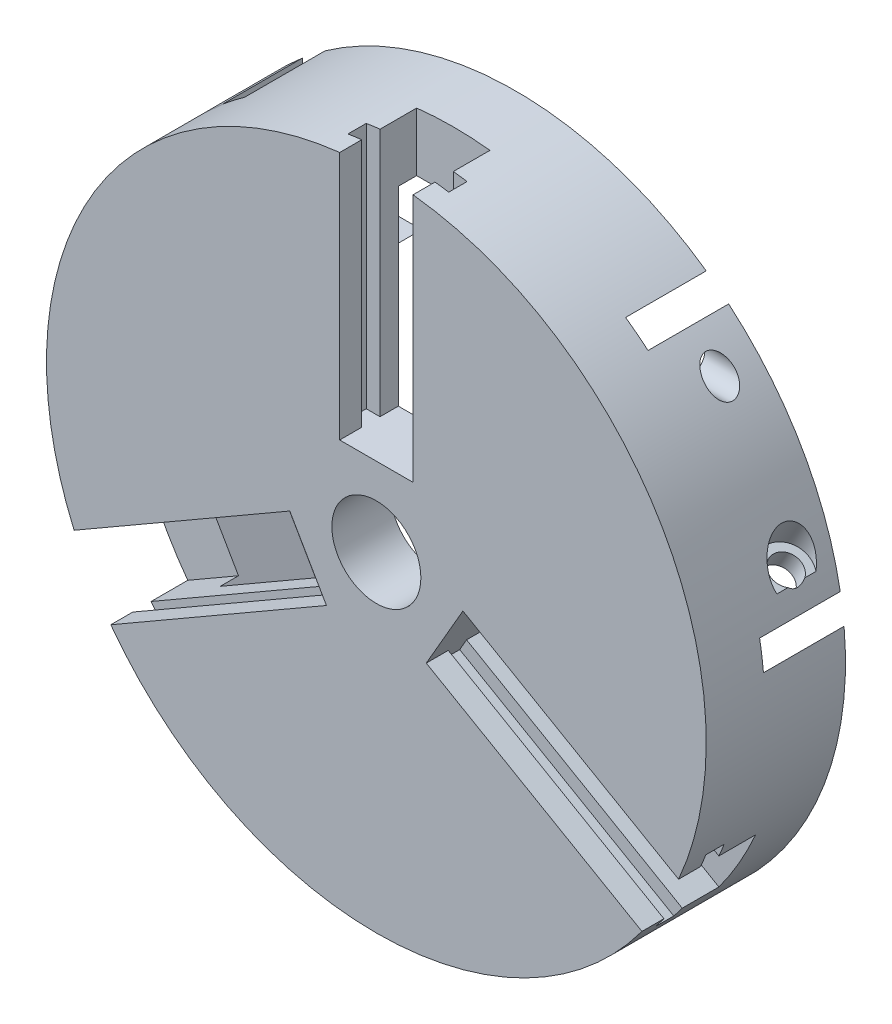
SolidWorks part; units mm, degrees
ref_plane "Front Plane" through (0, 0, 0) normal (0, 0, 1) x (1, 0, 0)
ref_plane "Top Plane" through (0, 0, 0) normal (0, 1, 0) x (1, 0, 0)
ref_plane "Right Plane" through (0, 0, 0) normal (1, 0, 0) x (0, 0, -1)
sketch "Sketch1" plane through (0, 0, 0) normal (0, 0, 1) x (1, 0, 0)
  circle A0 centre (0, 0) radius 180
  dimension "D1" = 360
extrude "Boss-Extrude1" add sketch "Sketch1" along normal blind 32
sketch "Sketch2" plane through (0, 0, 32) normal (0, 0, 1) x (1, 0, 0)
  line L0 (0, 188.4796) -> (0, 43) construction
  line L1 (20, 187.4154) -> (20, 43)
  line L2 (-20, 187.4154) -> (-20, 43)
  line L3 (-20, 43) -> (20, 43)
  arc A2 (20, 187.4154) -> (-20, 187.4154) centre (0, 0) ccw
  point P1 (0, 43)
  point P7 (0, 92.5)
  dimension "D1" = 43
  dimension "D3" = 40
extrude "Cut-Extrude1" cut sketch "Sketch2" against normal blind 40
pattern_circular "CirPattern1" count 3 over 360 about axis through (0, 0, 0) along (0, 0, 1) of "Cut-Extrude1"
sketch "Sketch3" plane through (37.2391, -21.5, 0) normal (0.866, -0.5, 0) x (0, 0, -1)
  line L0 (0, 0) -> (-32, 0) construction
  line L1 (-32, 20) -> (-32, -20) construction
  line L3 (-20, 27.5) -> (-10, 27.5)
  line L4 (-20, 27.5) -> (-20, -27.5)
  line L5 (-20, -27.5) -> (-10, -27.5)
  line L6 (-10, 27.5) -> (-10, -27.5)
  line L7 (-20, 27.5) -> (-10, -27.5) construction
  line L8 (-20, -27.5) -> (-10, 27.5) construction
  line L9 (0, 20) -> (0, 180) construction
  point P5 (-15, 0)
  dimension "D1" = 55
  dimension "D2" = 10
  dimension "D3" = 10
extrude "Cut-Extrude2" cut sketch "Sketch3" along normal blind 160
pattern_circular "CirPattern2" count 3 over 360 about axis through (0, 0, 0) along (0, 0, 1) of "Cut-Extrude2"
extrude "Cut-Extrude3" cut sketch "Sketch4" against normal blind 1
sketch "Sketch4" plane through (1185.0544, -482.7132, 0) normal (0, 0, -1) x (1, 0, 0)
  line L0 (-1236.3044, -571.4808) -> (-1301.3044, -571.4808)
  line L1 (-1301.3044, -571.4808) -> (-1301.3044, -620.1393)
  line L4 (-1133.8044, -571.4808) -> (-1068.8044, -571.4808)
  line L5 (-1068.8044, -571.4808) -> (-1068.8044, -620.1393)
  line L6 (-1301.3044, -620.1393) -> (-1068.8044, -620.1393) construction
  line L7 (-1236.3044, -393.9456) -> (-1203.8044, -337.6539)
  line L8 (-1203.8044, -337.6539) -> (-1245.9439, -313.3247)
  line L9 (-1287.5544, -482.7132) -> (-1320.0544, -539.0048)
  line L10 (-1320.0544, -539.0048) -> (-1362.1939, -514.6756)
  line L11 (-1082.5544, -482.7132) -> (-1050.0544, -539.0048)
  line L12 (-1050.0544, -539.0048) -> (-1007.9149, -514.6756)
  line L13 (-1133.8044, -393.9456) -> (-1166.3044, -337.6539)
  line L14 (-1166.3044, -337.6539) -> (-1124.1649, -313.3247)
  line L15 (-1236.3044, -571.4808) -> (-1185.0544, -482.7132) construction
  line L16 (-1185.0544, -482.7132) -> (-1133.8044, -571.4808) construction
  arc A0 (-1133.8044, -571.4808) -> (-1082.5544, -482.7132) centre (-1185.0544, -482.7132) ccw
  arc A1 (-1362.1939, -514.6756) -> (-1301.3044, -620.1393) centre (-1185.0544, -482.7132) ccw
  arc A4 (-1124.1649, -313.3247) -> (-1245.9439, -313.3247) centre (-1185.0544, -482.7132) ccw
  arc A5 (-1068.8044, -620.1393) -> (-1007.9149, -514.6756) centre (-1185.0544, -482.7132) ccw
  arc A6 (-1287.5544, -482.7132) -> (-1236.3044, -571.4808) centre (-1185.0544, -482.7132) ccw
  arc A7 (-1133.8044, -393.9456) -> (-1236.3044, -393.9456) centre (-1185.0544, -482.7132) ccw
sketch "Sketch5" plane through (0, 0, 0) normal (0, 0, -1) x (-1, 0, 0)
  line L0 (-116.25, 137.4261) -> (-116.25, 88.7676)
  line L1 (-102.5, 0) -> (-135, 56.2917)
  line L2 (-135, 56.2917) -> (-177.1395, 31.9624)
  line L3 (-116.25, 88.7676) -> (-51.25, 88.7676)
  arc A1 (-116.25, 137.4261) -> (-177.1395, 31.9624) centre (0, 0) ccw
  arc A2 (-51.25, 88.7676) -> (-102.5, 0) centre (0, 0) ccw
  arc A3 (-20, 178.8854) -> (-116.25, 137.4261) centre (0, 0) ccw construction
extrude "Boss-Extrude2" add sketch "Sketch5" along normal blind 44 and the other way blind 1 separate body
pattern_circular "CirPattern5" count 3 over 360 about axis through (0, 0, 0) along (0, 0, 1) of bodies 107
sketch "Sketch6" plane through (58.125, 100.6755, 0) normal (-0.5, -0.866, 0) x (0.866, -0.5, 0)
  line L0 (0, -23) -> (121.75, -23) construction
  line L1 (31.9624, -44) -> (137.4261, -44) construction
  circle A0 centre (121.75, -23) radius 8
  dimension "D3" = 16
  dimension "D1" = 121.75
  dimension "D2" = 21
extrude "Cut-Extrude4" cut sketch "Sketch6" against normal blind 51 and the other way blind 281
pattern_circular "CirPattern6" count 3 over 360 about axis through (0, 0, 32) along (0, 0, -1) of "Cut-Extrude4"
ref_plane "Plane1" through (63.125, -109.3357, 0) normal (-0.5, 0.866, 0) x (0.866, 0.5, 0)
sketch "Sketch7" plane through (63.125, -109.3357, 0) normal (-0.5, 0.866, 0) x (0.866, 0.5, 0)
  circle A0 centre (-121.75, 23) radius 12.5
  dimension "D1" = 25
extrude "Cut-Extrude5" cut sketch "Sketch7" against normal blind 30
pattern_circular "CirPattern7" count 3 over 360 about axis through (0, 0, 0) along (0, 0, 1) of "Cut-Extrude5"
sketch "Sketch10" plane through (0, 0, 0) normal (0, 0, -1) x (-1, 0, 0)
  line L0 (-179.2321, 16.6092) -> (-75.2321, -163.5241)
  line L1 (-47.2391, -4.1795) -> (-27.2391, -38.8205) construction
  line L2 (104, 146.9149) -> (-104, 146.9149)
  line L3 (75.2321, -163.5241) -> (179.2321, 16.6092)
  arc A0 (-177.1395, 31.9624) -> (-164.9193, -72.1222) centre (0, 0) ccw construction
  arc A1 (-144.9193, -106.7632) -> (-60.8895, -169.3885) centre (0, 0) ccw construction
  arc A2 (-179.2321, 16.6092) -> (-75.2321, -163.5241) centre (0, 0) ccw
  arc A3 (104, 146.9149) -> (-104, 146.9149) centre (0, 0) ccw
  arc A4 (75.2321, -163.5241) -> (179.2321, 16.6092) centre (0, 0) ccw
  point P17 (0, 0)
  dimension "D1" = 208
  dimension "D2" = 3
extrude "Boss-Extrude3" add sketch "Sketch10" along normal up to surface (44 mm away) up to face at (119.912, 69.2312, -44)
sketch "Sketch11" plane through (-37.2391, -21.5, 0) normal (-0.866, -0.5, 0) x (0, 0, 1)
  line L0 (0, -20) -> (10, -20) construction
  line L1 (0, 20) -> (-10, 20)
  line L2 (0, 20) -> (0, -20)
  line L3 (0, -20) -> (-10, -20)
  line L4 (-10, 20) -> (-10, -20)
  dimension "D1" = 10
extrude "Cut-Extrude8" cut sketch "Sketch11" along normal blind 160
sketch "Sketch12" plane through (0, 43, 0) normal (0, 1, 0) x (1, 0, 0)
  line L0 (20, 0) -> (20, -10) construction
  line L1 (-20, 0) -> (20, 0)
  line L2 (-20, 0) -> (-20, 10)
  line L3 (-20, 10) -> (20, 10)
  line L4 (20, 0) -> (20, 10)
  dimension "D1" = 10
extrude "Cut-Extrude9" cut sketch "Sketch12" along normal blind 160
sketch "Sketch13" plane through (37.2391, -21.5, 0) normal (0.866, -0.5, 0) x (0, 0, -1)
  line L1 (0, 20) -> (10, 20)
  line L2 (0, 20) -> (0, -20)
  line L3 (0, -20) -> (10, -20)
  line L4 (10, 20) -> (10, -20)
  dimension "D1" = 10
extrude "Cut-Extrude10" cut sketch "Sketch13" along normal blind 160
sketch "Sketch15" plane through (0, 0, 32) normal (0, 0, 1) x (1, 0, 0)
  circle A0 centre (0, 0) radius 24.2959
extrude "Cut-Extrude12" cut sketch "Sketch15" against normal blind 40
